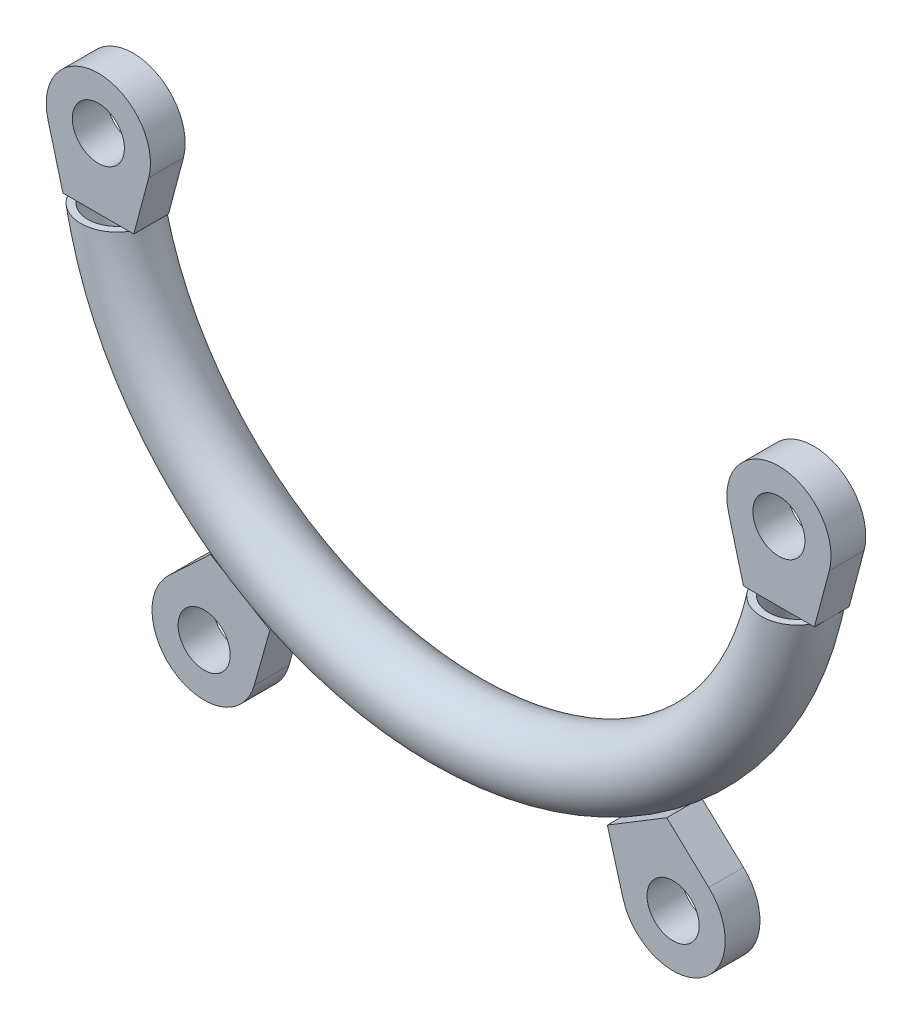
SolidWorks part; units mm, degrees
material "Q235-A"
ref_plane "前视基准面" through (0, 0, 0) normal (0, 0, 1) x (1, 0, 0)
ref_plane "上视基准面" through (0, 0, 0) normal (0, 1, 0) x (1, 0, 0)
ref_plane "右视基准面" through (0, 0, 0) normal (1, 0, 0) x (0, 0, -1)
sketch "草图1" plane through (0, 0, 0) normal (0, 0, 1) x (1, 0, 0)
  line L0 (0, 0) -> (0, -100) construction
  circle A0 centre (0, 0) radius 100
  dimension "D1" = 200
sketch "草图2" plane through (0, 0, 0) normal (1, 0, 0) x (0, 0, -1)
  line L0 (0, 100) -> (0, -100) construction
  line L1 (0, 0) -> (0, -100) construction
  circle A0 centre (0, -100) radius 10
  circle A1 centre (0, -100) radius 8
  dimension "D1" = 20
  dimension "D2" = 2
sweep "扫描1" add profiles "草图2" path "草图1"
sketch "草图3" plane through (0, 0, 0) normal (0, 0, 1) x (1, 0, 0)
  line L0 (-124.8211, -20) -> (0, -20)
  line L1 (0, -20) -> (127.8232, -20)
  line L2 (127.8232, -20) -> (127.8232, 142.661)
  line L3 (127.8232, 142.661) -> (-124.8211, 142.661)
  line L4 (-124.8211, 142.661) -> (-124.8211, -20)
  dimension "D1" = 20
extrude "切除-拉伸1" cut sketch "草图3" against normal through all both and the other way through all
sketch "草图4" plane through (0, 0, 0) normal (0, 0, 1) x (1, 0, 0)
  line L0 (-108.1665, -20) -> (-87.7496, -20) construction
  line L1 (-97.9581, -20) -> (-97.9581, 0) construction
  line L2 (-108.1665, -20) -> (-112.4555, -3.8502)
  line L3 (-87.7496, -20) -> (-83.4606, -3.8502)
  line L4 (-108.1665, -20) -> (-87.7496, -20)
  circle A0 centre (-97.9581, 0) radius 7.5
  arc A1 (-83.4606, -3.8502) -> (-112.4555, -3.8502) centre (-97.9581, 0) ccw
  arc A2 (-87.7496, -20) -> (87.7496, -20) centre (0, 0) ccw construction
  dimension "D1" = 15
  dimension "D2" = 30
  dimension "D3" = 20
extrude "凸台-拉伸1" add sketch "草图4" along normal mid plane 10
mirror "镜向1" about plane through (0, 0, 0) normal (1, 0, 0) of "凸台-拉伸1"
sketch "草图5" plane through (0, 0, 0) normal (0, 0, 1) x (1, 0, 0)
  line L0 (0, -110) -> (0, 0) construction
  line L1 (-67.5, -111.1024) -> (67.5, -111.1024) construction
  line L2 (-67.5, -111.1024) -> (0, 0) construction
  line L3 (-65.6617, -88.8174) -> (-48.569, -99.2021)
  line L4 (-65.6617, -88.8174) -> (-77.7594, -100.1597)
  line L5 (-48.569, -99.2021) -> (-53.0607, -115.1653)
  line L6 (65.6617, -88.8174) -> (77.7594, -100.1597)
  line L7 (65.6617, -88.8174) -> (48.569, -99.2021)
  line L8 (48.569, -99.2021) -> (53.0607, -115.1653)
  arc A0 (-108.1665, -20) -> (108.1665, -20) centre (0, 0) ccw construction
  circle A1 centre (-67.5, -111.1024) radius 7.5
  circle A2 centre (67.5, -111.1024) radius 7.5
  arc A3 (-77.7594, -100.1597) -> (-53.0607, -115.1653) centre (-67.5, -111.1024) ccw
  arc A4 (77.7594, -100.1597) -> (53.0607, -115.1653) centre (67.5, -111.1024) cw
  point P14 (-57.1154, -94.0097)
  dimension "D1" = 15
  dimension "D4" = 30
  dimension "D3" = 20
  dimension "D2" = 135
  dimension "D5" = 20
extrude "凸台-拉伸2" add sketch "草图5" along normal mid plane 10 separate body
